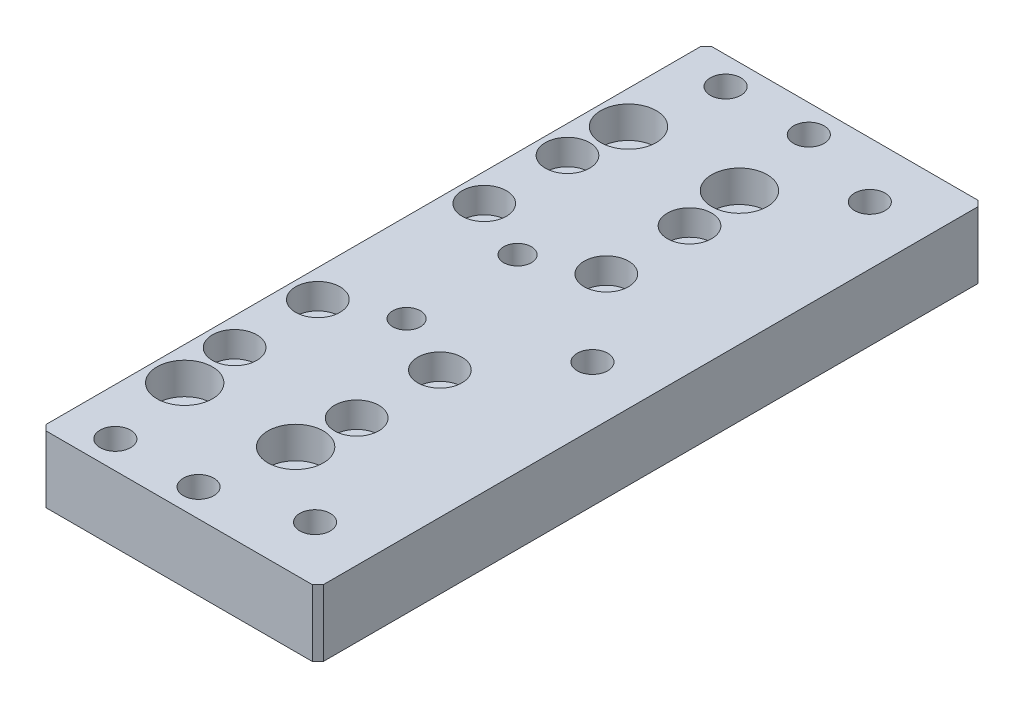
SolidWorks part; units mm, degrees
material "A6061"
ref_plane "前基準面" through (0, 0, 0) normal (0, 0, 1) x (1, 0, 0)
ref_plane "上基準面" through (0, 0, 0) normal (0, 1, 0) x (1, 0, 0)
ref_plane "右基準面" through (0, 0, 0) normal (1, 0, 0) x (0, 0, -1)
sketch "草图1" plane through (0, 0, 0) normal (0, 1, 0) x (1, 0, 0)
  line L1 (-25, -60) -> (25, -60)
  line L2 (-25, -60) -> (-25, 60)
  line L3 (-25, 60) -> (25, 60)
  line L4 (25, -60) -> (25, 60)
  line L5 (-25, -60) -> (25, 60) construction
  line L6 (-25, 60) -> (25, -60) construction
  point P0 (0, 0)
  dimension "D1" = 50
  dimension "D2" = 120
extrude "凸台-拉伸1" add sketch "草图1" along normal mid plane 12
sketch "草图2" plane through (0, 6, 0) normal (0, 1, 0) x (1, 0, 0)
  line L0 (-9, 53.978) -> (-9, 0) construction
  line L1 (-9, 0) -> (-25, 0) construction
  line L2 (-25, 60) -> (-25, -60) construction
  line L3 (-25, 60) -> (-25, -60) construction
  point P0 (2, 15)
  point P3 (-20, 30)
  point P16 (2, 30)
  point P17 (-20, 15)
  point P18 (-20, -15)
  point P19 (2, -30)
  point P20 (-20, -30)
  point P21 (2, -15)
  dimension "D1" = 22
  dimension "D2" = 15
  dimension "D3" = 45
  dimension "D4" = 16
hole_wizard "M4 六角圆柱头螺钉的柱形沉头孔1" positions "草图2" profile "草图3" counterbore size "M4" standard "GB" end condition through all
sketch "草图3" plane through (2, 6, -15) normal (1, 0, 0) x (0, 0, 1)
  line L0 (0, 0) -> (0, 12)
  line L1 (0, 12) -> (2.25, 12)
  line L3 (2.25, 12) -> (2.25, 4.6)
  line L4 (2.25, 4.6) -> (4, 4.6)
  line L5 (4, 4.6) -> (4, 0)
  line L7 (4, 0) -> (0, 0)
  line L11 (0, -6.35) -> (0, 107.95) construction
  dimension "通孔孔直径" = 4.5
  dimension "通孔孔深度" = 12
  dimension "柱形沉头孔直径" = 8
  dimension "柱形沉头孔深度" = 4.6
hole_wizard "M5 六角圆柱头螺钉的柱形沉头孔3" positions "草图7" profile "草图8" counterbore size "M5" standard "GB" end condition through all
sketch "草图7" plane through (0, -6, 0) normal (0, -1, 0) x (-1, 0, 0)
  line L0 (30.4873, 0) -> (9, 0) construction
  line L1 (9, 0) -> (9, 60.116) construction
  circle A0 centre (-2, 30) radius 2.25 construction
  circle A1 centre (20, 30) radius 2.25 construction
  point P0 (16.5, -55)
  point P14 (1.5, -55)
  point P15 (1.5, 55)
  point P16 (16.5, 55)
  dimension "D1" = 15
  dimension "D2" = 110
sketch "草图8" plane through (-16.5, -6, 55) normal (1, 0, 0) x (0, 0, -1)
  line L0 (0, 0) -> (0, 12)
  line L1 (0, 12) -> (2.75, 12)
  line L3 (2.75, 12) -> (2.75, 5.7)
  line L4 (2.75, 5.7) -> (4.75, 5.7)
  line L5 (4.75, 5.7) -> (4.75, 0)
  line L7 (4.75, 0) -> (0, 0)
  line L11 (0, -6.35) -> (0, 107.95) construction
  dimension "通孔孔直径" = 5.5
  dimension "通孔孔深度" = 12
  dimension "柱形沉头孔直径" = 9.5
  dimension "柱形沉头孔深度" = 5.7
sketch "草图9" plane through (0, 6, 0) normal (0, 1, 0) x (1, 0, 0)
  line L0 (-25, 0) -> (-9, 0) construction
  line L1 (-9, 0) -> (-9, 59.783) construction
  line L4 (-25, 60) -> (-25, -60) construction
  circle A0 centre (2, 30) radius 2.25 construction
  circle A1 centre (-20, 30) radius 2.25 construction
  point P0 (-9, 10)
  point P10 (-9, -10)
  dimension "D1" = 20
hole_wizard "M6 螺纹孔1" positions "草图9" profile "草图10" tap size "M6" standard "GB"
sketch "草图10" plane through (-9, 6, -10) normal (1, 0, 0) x (0, 0, 1)
  line L0 (0, 0) -> (0, 16.5022)
  line L1 (0, 16.5022) -> (2.5, 15)
  line L2 (2.5, 15) -> (2.5, 0)
  line L5 (2.5, 0) -> (0, 0)
  line L10 (0, 16.5022) -> (-2.5, 15) construction
  line L11 (0, -6.35) -> (0, 107.95) construction
  dimension "螺纹孔钻头直径" = 5
  dimension "螺纹孔钻头深度" = 15
  dimension "导头角度" = 118
cosmetic thread "孔螺纹线1" parameters "D1"=12, "D2"=6
cosmetic thread "孔螺纹线2" parameters "D1"=12, "D2"=6
sketch "草图11" plane through (0, 6, 0) normal (0, 1, 0) x (1, 0, 0)
  line L0 (-9, 62.5495) -> (-9, 0) construction
  line L1 (-9, 0) -> (-25, 0) construction
  line L2 (-25, 60) -> (-25, -60) construction
  circle A0 centre (-20, 30) radius 2.25 construction
  circle A1 centre (2, 30) radius 2.25 construction
  point P3 (1, 40)
  point P14 (1, -40)
  point P15 (-19, -40)
  point P16 (-19, 40)
  dimension "D1" = 20
  dimension "D2" = 80
hole_wizard "M5 六角圆柱头螺钉的柱形沉头孔1" positions "草图11" profile "草图12" counterbore size "M5" standard "GB" end condition through all
sketch "草图12" plane through (1, 6, -40) normal (1, 0, 0) x (0, 0, 1)
  line L0 (0, 0) -> (0, 12)
  line L1 (0, 12) -> (2.75, 12)
  line L3 (2.75, 12) -> (2.75, 5.7)
  line L4 (2.75, 5.7) -> (5, 5.7)
  line L5 (5, 5.7) -> (5, 0)
  line L7 (5, 0) -> (0, 0)
  line L11 (0, -6.35) -> (0, 107.95) construction
  dimension "通孔孔直径" = 5.5
  dimension "通孔孔深度" = 12
  dimension "柱形沉头孔直径" = 10
  dimension "柱形沉头孔深度" = 5.7
chamfer "倒角1" distance 1 angle 45 4 edges at (25, 0, -60) (-25, 0, -60) (25, 0, 60) (-25, 0, 60)
sketch "草图13" plane through (0, -6, 0) normal (0, -1, 0) x (-1, 0, 0)
  line L0 (0, 0) -> (-41.8329, 0) construction
  line L2 (-25, -59) -> (-25, 59) construction
  point P0 (-14.5, 50)
  point P7 (-14.5, 0)
  point P10 (-14.5, -50)
  dimension "D1" = 10.5
  dimension "D2" = 50
hole_wizard "M5 六角圆柱头螺钉的柱形沉头孔4" positions "草图13" profile "草图14" counterbore size "M5" standard "GB" end condition through all
sketch "草图14" plane through (14.5, -6, -50) normal (1, 0, 0) x (0, 0, -1)
  line L0 (0, 0) -> (0, 12)
  line L1 (0, 12) -> (2.75, 12)
  line L3 (2.75, 12) -> (2.75, 5.7)
  line L4 (2.75, 5.7) -> (5, 5.7)
  line L5 (5, 5.7) -> (5, 0)
  line L7 (5, 0) -> (0, 0)
  line L11 (0, -6.35) -> (0, 107.95) construction
  dimension "通孔孔直径" = 5.5
  dimension "通孔孔深度" = 12
  dimension "柱形沉头孔直径" = 10
  dimension "柱形沉头孔深度" = 5.7
